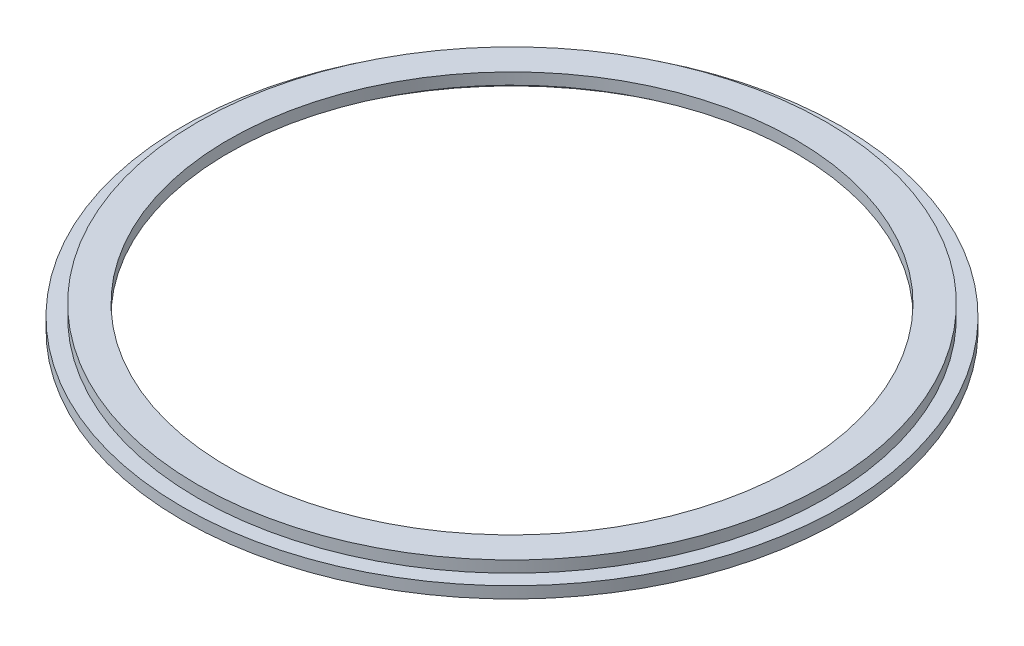
SolidWorks part; units mm, degrees
ref_plane "前视基准面" through (0, 0, 0) normal (0, 0, 1) x (1, 0, 0)
ref_plane "上视基准面" through (0, 0, 0) normal (0, 1, 0) x (1, 0, 0)
ref_plane "右视基准面" through (0, 0, 0) normal (1, 0, 0) x (0, 0, -1)
sketch "草图1" plane through (0, 0, 0) normal (0, 0, 1) x (1, 0, 0)
  line L0 (0, 0) -> (0, 27.5583) construction
  line L1 (-37, 0) -> (-41, 0)
  line L2 (-41, 0) -> (-41, -1.5)
  line L3 (-41, -1.5) -> (-43, -1.5)
  line L4 (-43, -1.5) -> (-43, -3)
  line L5 (-43, -3) -> (-39, -3)
  line L6 (-39, -3) -> (-39, -1.5)
  line L7 (-39, -1.5) -> (-37, -1.5)
  line L8 (-37, -1.5) -> (-37, 0)
  dimension "D1" = 74
  dimension "D2" = 78
  dimension "D3" = 1.5
  dimension "D4" = 2
revolve "旋转1" add sketch "草图1" angle 360 about L0
equation "\"图号代码1\"= \"图号代码\""
equation "\"名称代码2\"= \"名称代码\""
